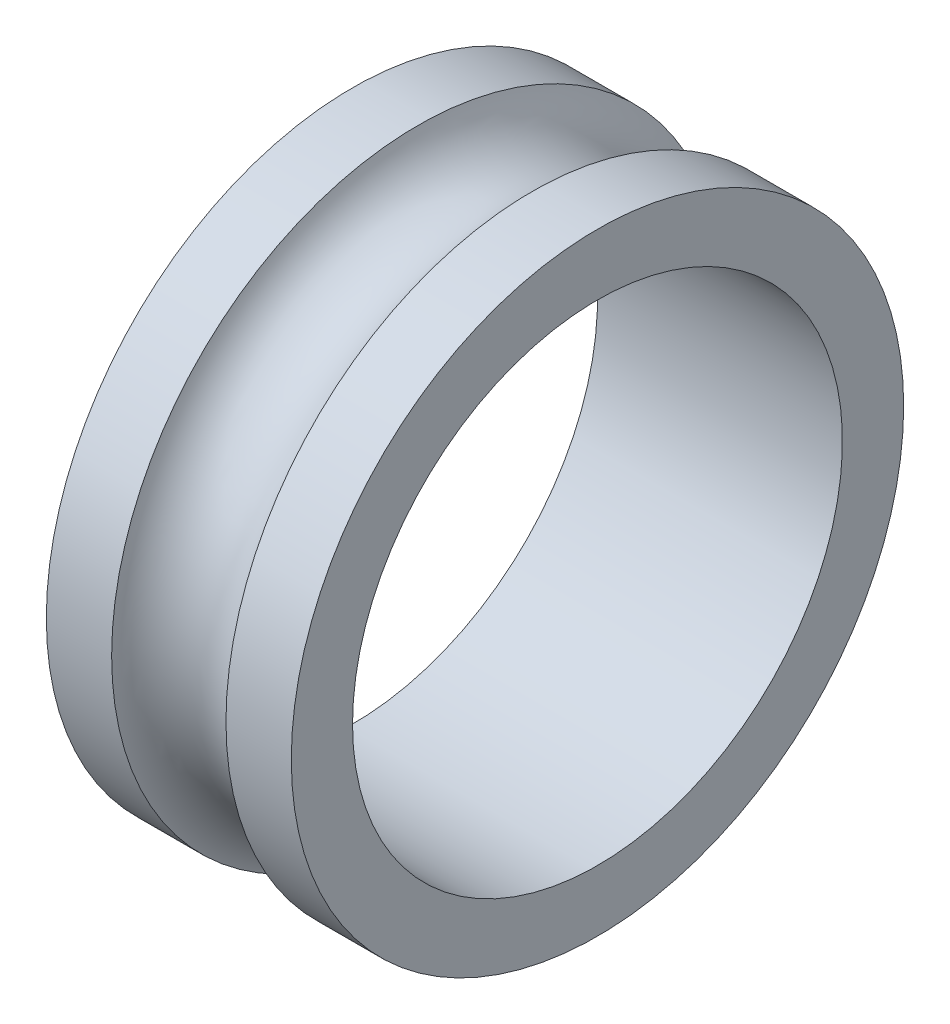
SolidWorks part; units mm, degrees
ref_plane "Front Plane" through (0, 0, 0) normal (0, 0, 1) x (1, 0, 0)
ref_plane "Top Plane" through (0, 0, 0) normal (0, 1, 0) x (1, 0, 0)
ref_plane "Right Plane" through (0, 0, 0) normal (1, 0, 0) x (0, 0, -1)
sketch "Sketch1" plane through (0, 0, 0) normal (0, 0, 1) x (1, 0, 0)
  line L0 (0, 0) -> (63.3398, 0) construction
  line L1 (0, 6) -> (0, 7.5)
  line L2 (0, 7.5) -> (1.6, 7.5)
  line L3 (1.6, 7.5) -> (1.6, 6.5) construction
  line L4 (1.6, 6.5) -> (4.4, 6.5) construction
  line L5 (4.4, 6.5) -> (4.4, 7.5) construction
  line L6 (4.4, 7.5) -> (6, 7.5)
  line L7 (6, 7.5) -> (6, 6)
  line L8 (0, 6) -> (6, 6)
  arc A0 (1.6, 7.5) -> (4.4, 7.5) centre (3, 7.98) ccw
  dimension "D1" = 6
  dimension "D2" = 2.8
  dimension "D3" = 1.6
  dimension "D4" = 1
  dimension "D5" = 0
  dimension "D6" = 7.5
  dimension "D7" = 12
revolve "Revolve1" add sketch "Sketch1" angle 360 about L0
